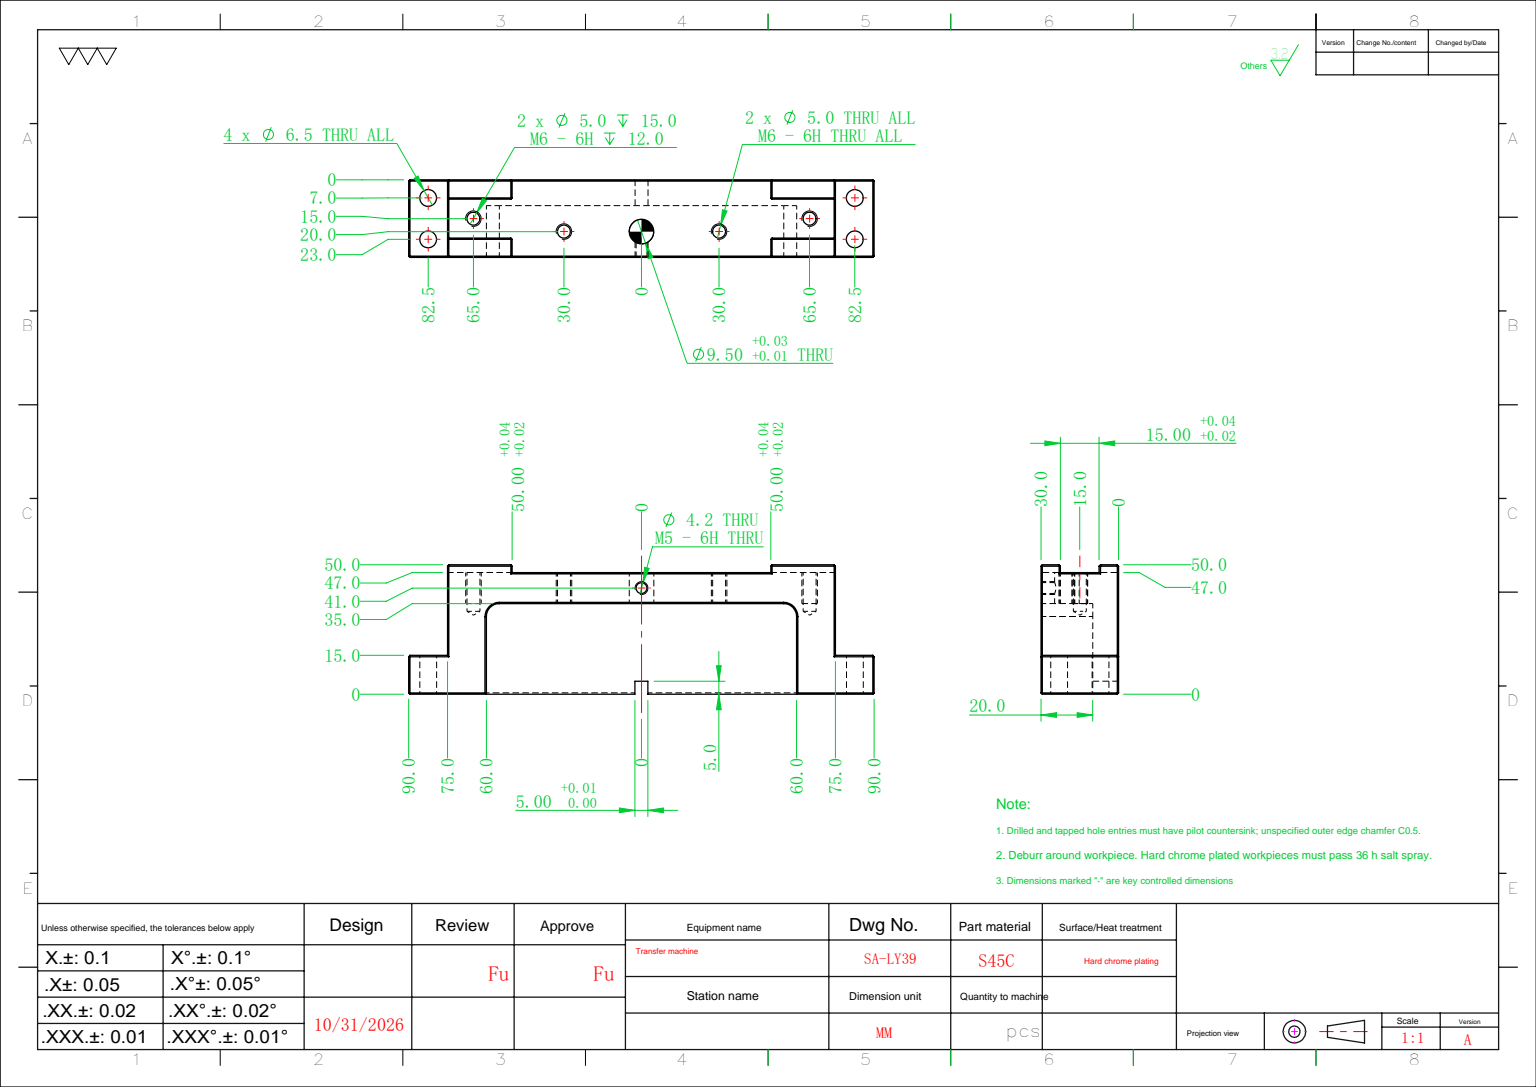
from build123d import *

# Parameters (mm, degrees)
SKETCH_1_W              = 150
SKETCH_1_H              = 30
EXTRUDE_1_DEPTH         = 50
SKETCH_3_W              = 120
SKETCH_3_H              = 35
CUT_EXTRUDE_2_DEPTH     = 20
SKETCH_4_W              = 100
SKETCH_4_H              = 3
CUT_EXTRUDE_3_DEPTH     = 96
SKETCH_5_W              = 150
SKETCH_5_H              = 15
CUT_EXTRUDE_4_DEPTH     = 3
FILLET_1_R              = 5
HOLE_WIZARD_M6_1_D      = 5
SKETCH_11_R             = 4.75
CUT_EXTRUDE_6_DEPTH     = 85.113019206
HOLE_WIZARD_M5_1_REACH  = 97
HOLE_WIZARD_M5_1_BORE_R = 2.1
HOLE_WIZARD_M6_2_D      = 5
HOLE_WIZARD_M6_2_DEPTH  = 15
HOLE_WIZARD_M6_2_TIP    = 1.502151548
SKETCH_18_W             = 15
SKETCH_18_H             = 15
EXTRUDE_2_DEPTH         = 30
HOLE_WIZARD_6_5_6_5_1_D = 6.5
SKETCH_21_W             = 5
SKETCH_21_H             = 10
CUT_EXTRUDE_7_DEPTH     = 105.880884836
CHAMFER_1_SIZE          = 0.5


with BuildPart() as part:
    # 草图1 → 凸台-拉伸1 (new body)
    with BuildSketch(Plane.XY):
        Rectangle(SKETCH_1_W, SKETCH_1_H)
    extrude(amount=EXTRUDE_1_DEPTH)

    # 草图3 → 切除-拉伸2 (cut)
    with BuildSketch(Plane.XZ.offset(15)):
        with Locations((0, 17.5)):
            Rectangle(SKETCH_3_W, SKETCH_3_H)
    extrude(amount=-CUT_EXTRUDE_2_DEPTH, mode=Mode.SUBTRACT)

    # 草图4 → 切除-拉伸3 (cut, through all)
    with BuildSketch(Plane.XZ.offset(15)):
        with Locations((0, 48.5)):
            Rectangle(SKETCH_4_W, SKETCH_4_H)
    extrude(amount=-CUT_EXTRUDE_3_DEPTH, mode=Mode.SUBTRACT)

    # 草图5 → 切除-拉伸4 (cut)
    with BuildSketch(Plane.XY.offset(50)):
        Rectangle(SKETCH_5_W, SKETCH_5_H)
    extrude(amount=-CUT_EXTRUDE_4_DEPTH, mode=Mode.SUBTRACT)

    # 圆角1
    fillet_1_edges = [part.edges().sort_by_distance(p)[0] for p in [
        (-60, -5, 35),
        (60, -5, 35),
    ]]
    fillet(fillet_1_edges, radius=FILLET_1_R)

    # M6 螺纹孔1 (through all)
    with Locations(Plane(origin=(0, 0, 35), x_dir=(-1, 0, 0), z_dir=(0, 0, -1))):
        with Locations((30, -5), (-30, -5)):
            Hole(HOLE_WIZARD_M6_1_D / 2)

    # 草图11 → 切除-拉伸6 (cut, through all)
    with BuildSketch(Plane(origin=(0, 0, 35), x_dir=(-1, 0, 0), z_dir=(0, 0, -1))):
        with Locations((0, -5)):
            Circle(SKETCH_11_R)
    extrude(amount=-CUT_EXTRUDE_6_DEPTH, mode=Mode.SUBTRACT)

    # M5 螺纹孔1 bore → M5 螺纹孔1 (cut, up to next)
    with BuildSketch(Plane(origin=(0, -15, 0), x_dir=(-1, 0, 0), z_dir=(0, -1, 0)), mode=Mode.PRIVATE) as hole_wizard_m5_1_sk1:
        with Locations((0, -41)):
            Circle(HOLE_WIZARD_M5_1_BORE_R)
    hole_wizard_m5_1_tool1 = extrude(hole_wizard_m5_1_sk1.sketch, amount=-HOLE_WIZARD_M5_1_REACH, mode=Mode.PRIVATE) & part.part
    add(hole_wizard_m5_1_tool1.solids().sort_by_distance((0, -15, 41))[0], mode=Mode.SUBTRACT)

    # M6 螺纹孔2
    with Locations(Plane.XY.offset(47)):
        with Locations((-65, 0), (65, 0)):
            Hole(HOLE_WIZARD_M6_2_D / 2, depth=HOLE_WIZARD_M6_2_DEPTH)
            with Locations((0, 0, -(HOLE_WIZARD_M6_2_DEPTH + HOLE_WIZARD_M6_2_TIP / 2))):  # 118° drill point
                Cone(0, HOLE_WIZARD_M6_2_D / 2, HOLE_WIZARD_M6_2_TIP, mode=Mode.SUBTRACT)

    # 草图18 → 凸台-拉伸2 (add)
    with BuildSketch(Plane.XZ.offset(15)):
        with Locations((-82.5, 7.5)):
            Rectangle(SKETCH_18_W, SKETCH_18_H)
        with Locations((82.5, 7.5)):
            Rectangle(SKETCH_18_W, SKETCH_18_H)
    extrude(amount=-EXTRUDE_2_DEPTH)

    # Ø6.5 (6.5) 直径孔1 (through all)
    with Locations(Plane.XY.offset(15)):
        with Locations((-82.5, 8), (-82.5, -8), (82.5, -8), (82.5, 8)):
            Hole(HOLE_WIZARD_6_5_6_5_1_D / 2)

    # 草图21 → 切除-拉伸7 (cut, through all)
    with BuildSketch(Plane.XZ.offset(-5)):
        Rectangle(SKETCH_21_W, SKETCH_21_H)
    extrude(amount=-CUT_EXTRUDE_7_DEPTH, mode=Mode.SUBTRACT)

    # 倒角1
    chamfer_1_edges = [part.edges().sort_by_distance(p)[0] for p in [
        (-90, 0, 0),
        (-90, 0, 15),
        (-82.5, -15, 15),
        (-90, -15, 7.5),
        (-90, 15, 7.5),
        (-82.5, 15, 15),
        (-75, 11.25, 50),
        (90, 0, 0),
        (90, 0, 15),
        (90, -15, 7.5),
        (82.5, -15, 15),
        (82.5, 15, 15),
        (90, 15, 7.5),
        (75, -15, 0),
        (-62.5, -15, 50),
        (-46.25, 15, 0),
        (60, -15, 15),
        (-62.5, 15, 50),
        (62.5, -15, 50),
        (-50, 15, 48.5),
        (-50, 11.25, 50),
        (50, 15, 48.5),
        (50, 11.25, 50),
        (0, 15, 47),
        (-50, -15, 48.5),
        (0, -15, 47),
        (50, -15, 48.5),
        (50, -11.25, 50),
        (-50, -11.25, 50),
        (75, -11.25, 50),
        (-75, -15, 0),
        (75, 11.25, 50),
        (-75, -11.25, 50),
        (-62.5, 7.5, 50),
        (-62.5, -7.5, 50),
        (62.5, -7.5, 50),
        (62.5, 7.5, 50),
        (-50, -7.5, 48.5),
        (50, -7.5, 48.5),
        (75, -7.5, 48.5),
        (46.25, 15, 0),
        (-50, 7.5, 48.5),
        (-75, 7.5, 48.5),
        (50, 7.5, 48.5),
        (75, 0, 47),
        (75, 7.5, 48.5),
        (-75, 0, 47),
        (-75, -7.5, 48.5),
        (-60, -15, 15),
        (0, -15, 35),
        (75, -15, 32.5),
        (-75, -15, 32.5),
        (-75, 15, 32.5),
        (-58.535533906, -15, 33.535533906),
        (58.535533906, -15, 33.535533906),
        (75, 15, 32.5),
        (62.5, 15, 50),
    ]]
    chamfer(chamfer_1_edges, length=CHAMFER_1_SIZE)


solid = part.part
